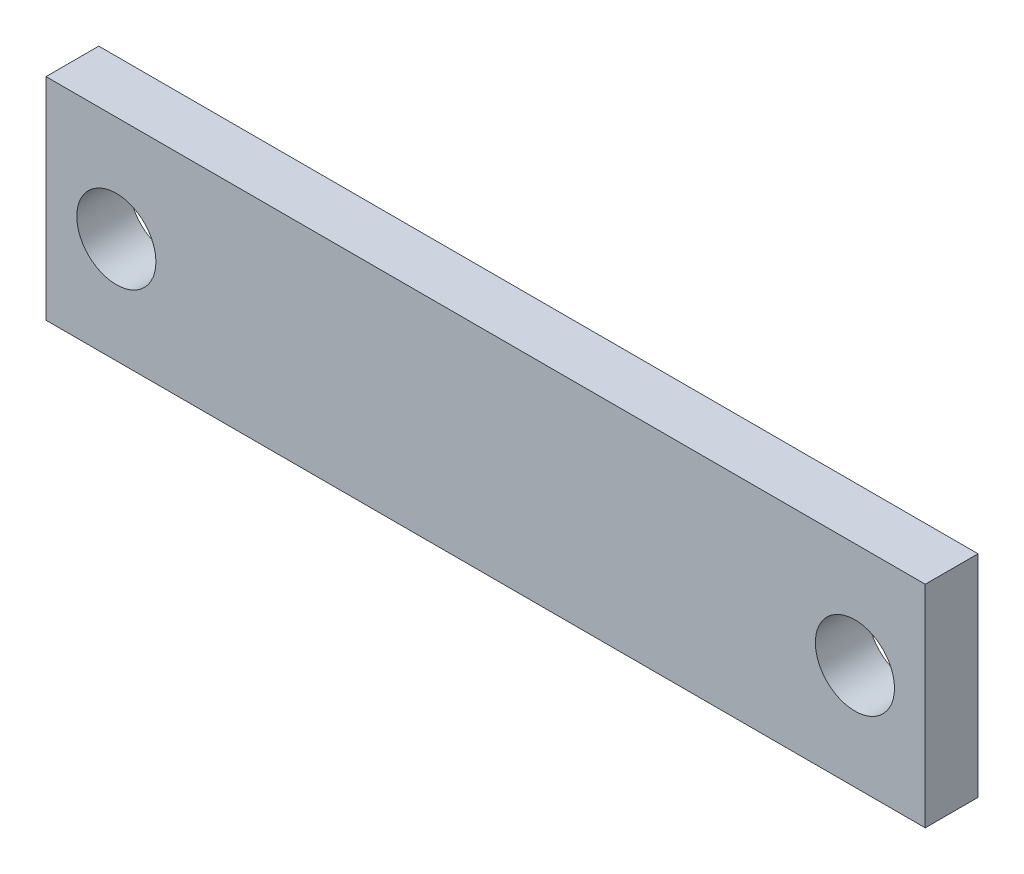
SolidWorks part; units mm, degrees
ref_plane "前视基准面" through (0, 0, 0) normal (0, 0, 1) x (1, 0, 0)
ref_plane "上视基准面" through (0, 0, 0) normal (0, 1, 0) x (1, 0, 0)
ref_plane "右视基准面" through (0, 0, 0) normal (1, 0, 0) x (0, 0, -1)
sketch "草图1" plane through (0, 0, 0) normal (0, 0, 1) x (1, 0, 0)
  line L1 (-25, -6) -> (25, -6)
  line L2 (-25, -6) -> (-25, 6)
  line L3 (-25, 6) -> (25, 6)
  line L4 (25, -6) -> (25, 6)
  line L5 (-25, -6) -> (25, 6) construction
  line L6 (-25, 6) -> (25, -6) construction
  circle A0 centre (-21, 0) radius 2.25
  circle A1 centre (21, 0) radius 2.25
  point P0 (0, 0)
  dimension "D3" = 4.5
  dimension "D1" = 50
  dimension "D2" = 12
  dimension "D4" = 4
  dimension "D5" = 4
extrude "凸台-拉伸1" add sketch "草图1" along normal mid plane 3
